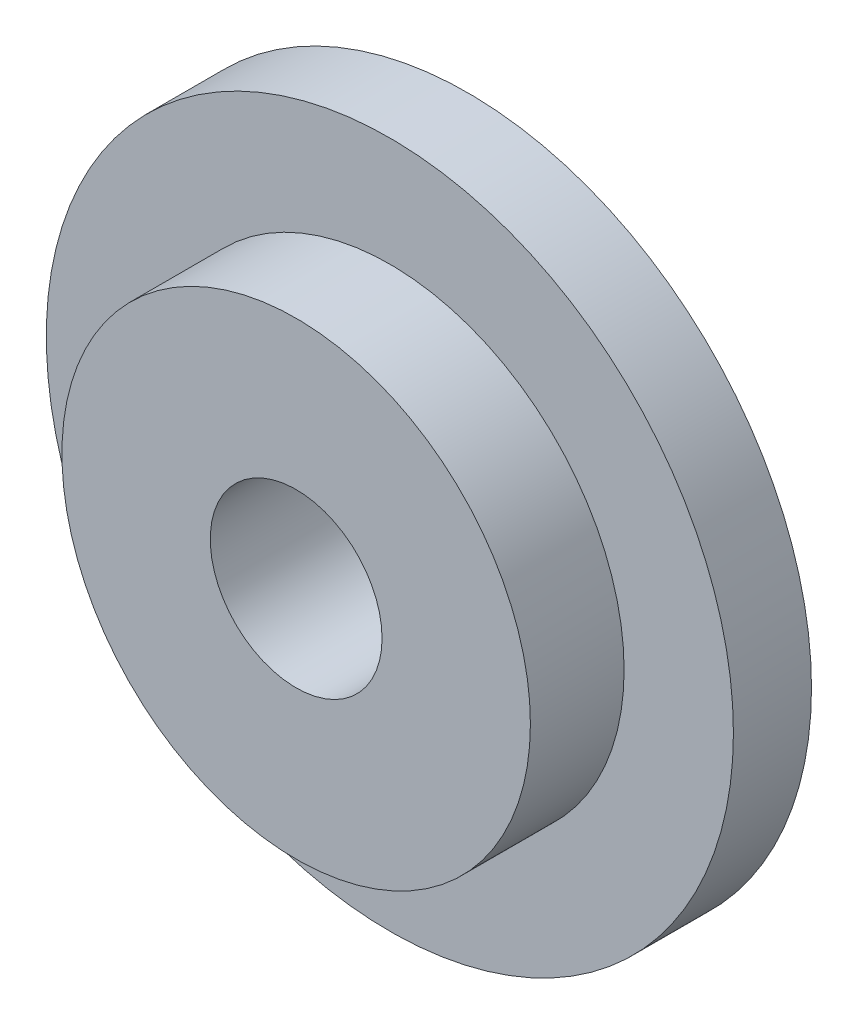
SolidWorks part; units mm, degrees
ref_plane "Front Plane" through (0, 0, 0) normal (0, 0, 1) x (1, 0, 0)
ref_plane "Top Plane" through (0, 0, 0) normal (0, 1, 0) x (1, 0, 0)
ref_plane "Right Plane" through (0, 0, 0) normal (1, 0, 0) x (0, 0, -1)
other "Configuration Table"
sketch "Sketch1" plane through (0, 0, 0) normal (1, 0, 0) x (0, 0, -1)
  line L0 (-17.9084, 0) -> (12.0947, 0) construction
  line L1 (0, 15) -> (0, 5.5)
  line L2 (0, 5.5) -> (9, 5.5)
  line L3 (9, 5.5) -> (11, 8.9641)
  line L4 (11, 8.9641) -> (11, 22)
  line L5 (11, 22) -> (6, 22)
  line L6 (6, 22) -> (6, 15)
  line L7 (6, 15) -> (0, 15)
  dimension "D1" = 11
  dimension "D2" = 30
  dimension "D3" = 44
  dimension "D4" = 5
  dimension "D5" = 11
  dimension "D6" = 60
  dimension "D7" = 2
revolve "Revolve1" add sketch "Sketch1" angle 360 about L0
